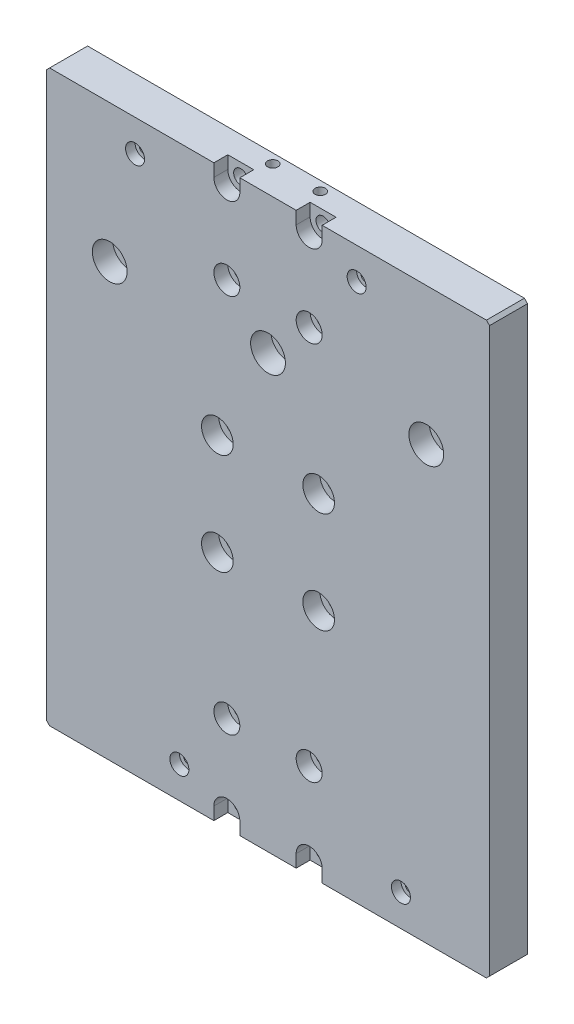
from build123d import *

# Parameters (mm, degrees)
SKETCH1_W                                           = 140
SKETCH1_H                                           = 180
BOSS_EXTRUDE1_DEPTH                                 = 6
CBORE_FOR_M4_HEX_SOCKET_HEAD_CAP_SCREW2_D           = 4.5
CBORE_FOR_M4_HEX_SOCKET_HEAD_CAP_SCREW2_CBORE_D     = 8.2
CBORE_FOR_M4_HEX_SOCKET_HEAD_CAP_SCREW2_CBORE_DEPTH = 4.4
SIZE_MM_DOWEL_HOLE_1_D                              = 5
SIZE_MM_DOWEL_HOLE_1_DEPTH                          = 10
SIZE_MM_DOWEL_HOLE_1_TIP                            = 1.502151548
CBORE_FOR_M5_HEX_SOCKET_HEAD_CAP_SCREW1_D           = 5.5
CBORE_FOR_M5_HEX_SOCKET_HEAD_CAP_SCREW1_CBORE_D     = 10
CBORE_FOR_M5_HEX_SOCKET_HEAD_CAP_SCREW1_CBORE_DEPTH = 5.4
SKETCH10_W                                          = 8.2
SKETCH10_H                                          = 4
CUT_EXTRUDE1_DEPTH                                  = 4.4
M4_TAPPED_HOLE1_D                                   = 3.3
M4_TAPPED_HOLE1_DEPTH                               = 15.5
M4_TAPPED_HOLE1_TIP                                 = 0.991420021
SIZE_MM_DOWEL_HOLE_2_D                              = 6
SIZE_MM_DOWEL_HOLE_2_DEPTH                          = 3
CBORE_FOR_M3_HEX_SOCKET_HEAD_CAP_SCREW1_D           = 3.4
CBORE_FOR_M3_HEX_SOCKET_HEAD_CAP_SCREW1_CBORE_D     = 6.5
CBORE_FOR_M3_HEX_SOCKET_HEAD_CAP_SCREW1_CBORE_DEPTH = 3.4
CHAMFER1_SIZE                                       = 1
CBORE_FOR_M6_HEX_SOCKET_HEAD_CAP_SCREW1_D           = 6.6
CBORE_FOR_M6_HEX_SOCKET_HEAD_CAP_SCREW1_CBORE_D     = 11
CBORE_FOR_M6_HEX_SOCKET_HEAD_CAP_SCREW1_CBORE_DEPTH = 6.4


with BuildPart() as part:
    # Sketch1 → Boss-Extrude1 (new, symmetric)
    with BuildSketch(Plane.XY):
        Rectangle(SKETCH1_W, SKETCH1_H)
    extrude(amount=BOSS_EXTRUDE1_DEPTH, both=True)

    # CBORE for M4 Hex Socket Head Cap Screw2 (through all)
    with Locations(Plane.XY.offset(6)):
        with Locations((13, -60), (-13, -60), (-13, -86), (13, -86), (-13, 86), (13, 86), (-13, 60), (13, 60)):
            CounterBoreHole(CBORE_FOR_M4_HEX_SOCKET_HEAD_CAP_SCREW2_D / 2, CBORE_FOR_M4_HEX_SOCKET_HEAD_CAP_SCREW2_CBORE_D / 2, CBORE_FOR_M4_HEX_SOCKET_HEAD_CAP_SCREW2_CBORE_DEPTH)

    # Size mm dowel hole 1
    with Locations(Plane(origin=(0, 0, -6), x_dir=(-1, 0, 0), z_dir=(0, 0, -1))):
        with Locations((14.7, -51), (-14.7, -51), (14.7, 53.5), (-14.7, 53.5)):
            Hole(SIZE_MM_DOWEL_HOLE_1_D / 2, depth=SIZE_MM_DOWEL_HOLE_1_DEPTH)
            with Locations((0, 0, -(SIZE_MM_DOWEL_HOLE_1_DEPTH + SIZE_MM_DOWEL_HOLE_1_TIP / 2))):  # 118° drill point
                Cone(0, SIZE_MM_DOWEL_HOLE_1_D / 2, SIZE_MM_DOWEL_HOLE_1_TIP, mode=Mode.SUBTRACT)

    # CBORE for M5 Hex Socket Head Cap Screw1 (through all)
    with Locations(Plane.XY.offset(6)):
        with Locations((16, 16), (-16, 16), (-16, -16), (16, -16)):
            CounterBoreHole(CBORE_FOR_M5_HEX_SOCKET_HEAD_CAP_SCREW1_D / 2, CBORE_FOR_M5_HEX_SOCKET_HEAD_CAP_SCREW1_CBORE_D / 2, CBORE_FOR_M5_HEX_SOCKET_HEAD_CAP_SCREW1_CBORE_DEPTH)

    # Sketch10 → Cut-Extrude1 (cut)
    with BuildSketch(Plane.XY.offset(6)):
        with Locations((-13, 88)):
            Rectangle(SKETCH10_W, SKETCH10_H)
        with Locations((13, 88)):
            Rectangle(SKETCH10_W, SKETCH10_H)
        with Locations((-13, -88)):
            Rectangle(SKETCH10_W, SKETCH10_H)
        with Locations((13, -88)):
            Rectangle(SKETCH10_W, SKETCH10_H)
    extrude(amount=-CUT_EXTRUDE1_DEPTH, mode=Mode.SUBTRACT)

    # M4 Tapped Hole1
    with Locations(Plane(origin=(0, 90, 0), x_dir=(1, 0, 0), z_dir=(0, 1, 0))):
        with Locations((-7.5, 3), (7.5, 3)):
            Hole(M4_TAPPED_HOLE1_D / 2, depth=M4_TAPPED_HOLE1_DEPTH)
            with Locations((0, 0, -(M4_TAPPED_HOLE1_DEPTH + M4_TAPPED_HOLE1_TIP / 2))):  # 118° drill point
                Cone(0, M4_TAPPED_HOLE1_D / 2, M4_TAPPED_HOLE1_TIP, mode=Mode.SUBTRACT)

    # Size mm dowel hole 2
    with Locations(Plane.XY.offset(6)):
        with Locations((28, 80), (-42, 80), (42, -80), (-28, -80)):
            Hole(SIZE_MM_DOWEL_HOLE_2_D / 2, depth=SIZE_MM_DOWEL_HOLE_2_DEPTH)

    # CBORE for M3 Hex Socket Head Cap Screw1 (through all)
    with Locations(Plane(origin=(0, 0, -6), x_dir=(-1, 0, 0), z_dir=(0, 0, -1))):
        with Locations((-28, 80), (42, 80), (28, -80), (-42, -80)):
            CounterBoreHole(CBORE_FOR_M3_HEX_SOCKET_HEAD_CAP_SCREW1_D / 2, CBORE_FOR_M3_HEX_SOCKET_HEAD_CAP_SCREW1_CBORE_D / 2, CBORE_FOR_M3_HEX_SOCKET_HEAD_CAP_SCREW1_CBORE_DEPTH)

    # Chamfer1
    chamfer1_edges = [part.edges().sort_by_distance(p)[0] for p in [
        (70, -90, 0),
        (-70, -90, 0),
        (-70, 90, 0),
        (70, 90, 0),
    ]]
    chamfer(chamfer1_edges, length=CHAMFER1_SIZE)

    # CBORE for M6 Hex Socket Head Cap Screw1 (through all)
    with Locations(Plane.XY.offset(6)):
        with Locations((-50, 46.5), (0, 46.5), (50, 46.5)):
            CounterBoreHole(CBORE_FOR_M6_HEX_SOCKET_HEAD_CAP_SCREW1_D / 2, CBORE_FOR_M6_HEX_SOCKET_HEAD_CAP_SCREW1_CBORE_D / 2, CBORE_FOR_M6_HEX_SOCKET_HEAD_CAP_SCREW1_CBORE_DEPTH)


solid = part.part
